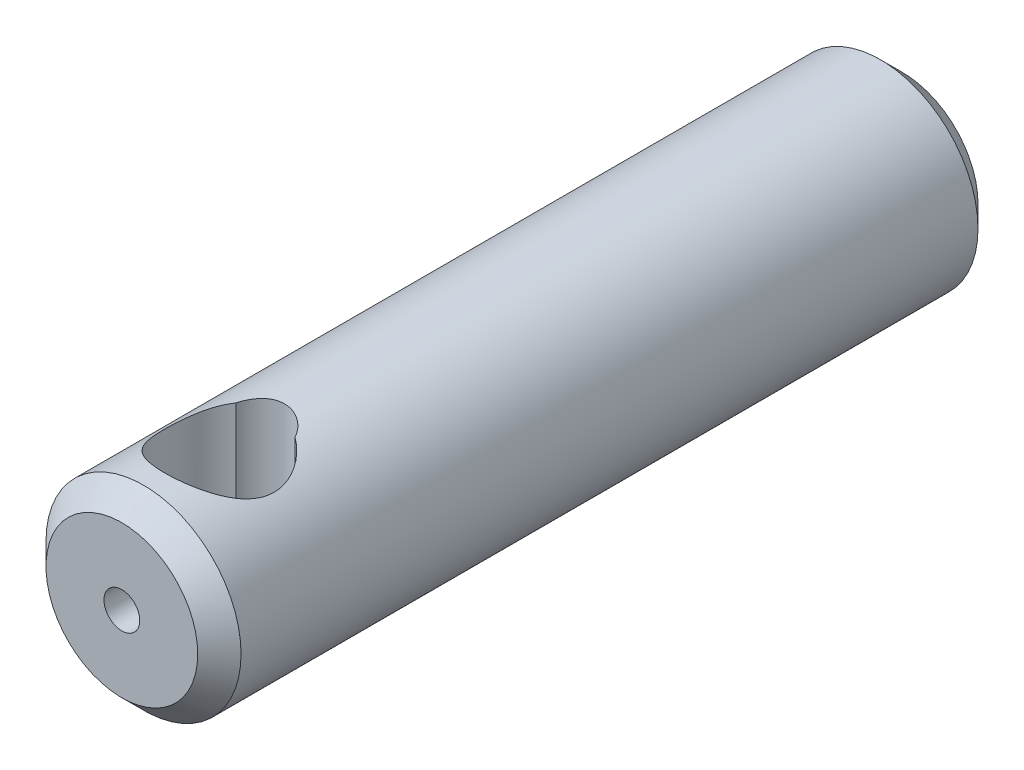
SolidWorks part; units mm, degrees
material "304"
ref_plane "Front Plane" through (0, 0, 0) normal (0, 0, 1) x (1, 0, 0)
ref_plane "Top Plane" through (0, 0, 0) normal (0, 1, 0) x (1, 0, 0)
ref_plane "Right Plane" through (0, 0, 0) normal (1, 0, 0) x (0, 0, -1)
sketch "Sketch1" plane through (0, 0, 0) normal (0, 0, 1) x (1, 0, 0)
  circle A0 centre (0, 0) radius 9
  dimension "D1" = 18
extrude "Boss-Extrude1" add sketch "Sketch1" along normal blind 72
sketch "Sketch2" plane through (0, 0, 0) normal (0, 1, 0) x (1, 0, 0)
  line L0 (-9, -72) -> (9, -72) construction
  arc A0 (-2.727, -58.7496) -> (2.727, -58.7496) centre (0, -63) ccw
  arc A2 (2.727, -58.7496) -> (-2.727, -58.7496) centre (0, -60) ccw
  dimension "D1" = 5.05
  dimension "D2" = 9
  dimension "D3" = 12
  dimension "D4" = 6
extrude "Cut-Extrude1" cut sketch "Sketch2" against normal through all and the other way through all
hole_wizard "M4 Tapped Hole1" positions "Sketch4" profile "Sketch3" tap size "M4" standard "GB"
sketch "Sketch4" plane through (0, 0, 72) normal (0, 0, 1) x (1, 0, 0)
  point P0 (0, 0)
sketch "Sketch3" plane through (0, 0, 72) normal (1, 0, 0) x (0, -1, 0)
  line L0 (0, 0) -> (0, 3.95)
  line L1 (0, 3.95) -> (1.65, 3.95)
  line L2 (1.65, 3.95) -> (1.65, 0)
  line L5 (1.65, 0) -> (0, 0)
  line L11 (0, -6.35) -> (0, 107.95) construction
  dimension "通孔螺纹孔钻头直径" = 3.3
  dimension "通孔螺纹孔钻头深度" = 3.95
cosmetic thread "Cosmetic Thread3" parameters "D2"=4
chamfer "Chamfer1" distance 2 angle 45 2 edges at (9, 0, 0) (9, 0, 72)
